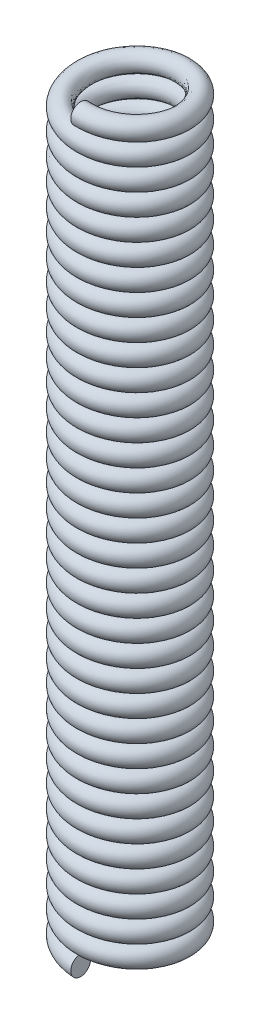
from build123d import *

# Parameters (mm, degrees)
SWEEP1_PITCH  = 0.55
SWEEP1_HEIGHT = 18.7
SWEEP1_RADIUS = 1.25
SKETCH2_R     = 0.25


with BuildPart() as part:
    # Sweep1: sweep along a helix
    with BuildLine() as sweep1_path:
        Helix(SWEEP1_PITCH, SWEEP1_HEIGHT, SWEEP1_RADIUS, center=(0, 0, 0), direction=(0, 1, 0), lefthand=True)
    # Sketch2 → Sweep1 (sweep)
    with BuildSketch(Plane(origin=(0, 0, 0), x_dir=(0, 0, -1), z_dir=(1, 0, 0))):
        with Locations((-1.25, 0)):
            Circle(SKETCH2_R)
    sweep(path=sweep1_path.line, is_frenet=True)


solid = part.part
